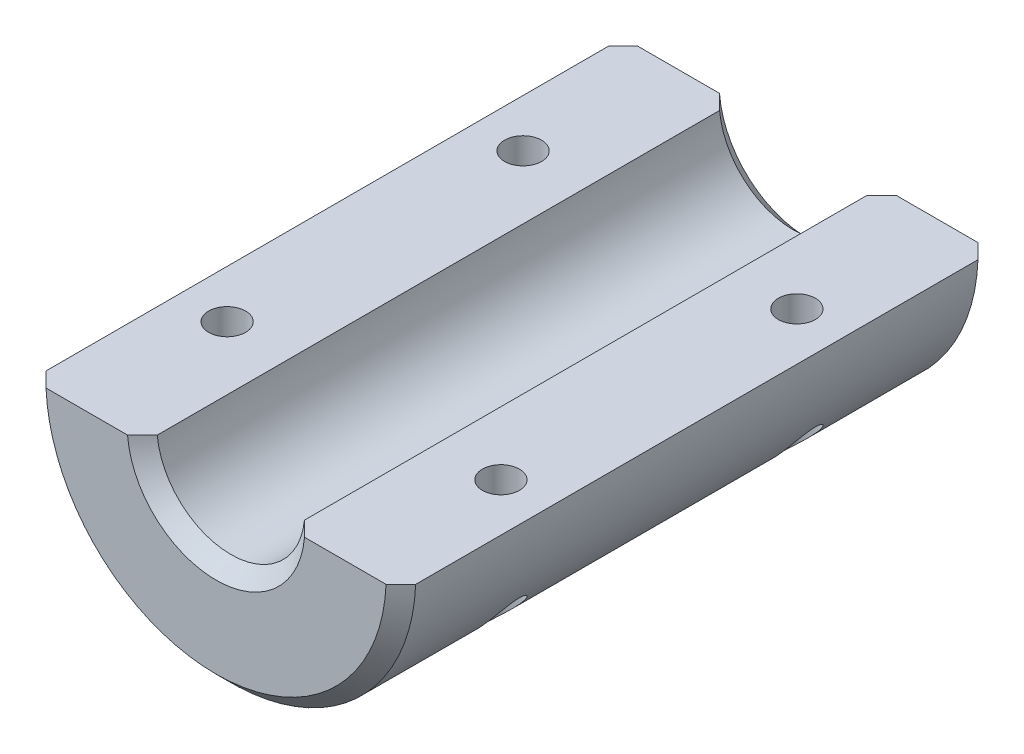
SolidWorks part; units mm, degrees
material "6061-T4 (SS)"
ref_plane "前视基准面" through (0, 0, 0) normal (0, 0, 1) x (1, 0, 0)
ref_plane "上视基准面" through (0, 0, 0) normal (0, 1, 0) x (1, 0, 0)
ref_plane "右视基准面" through (0, 0, 0) normal (1, 0, 0) x (0, 0, -1)
sketch "草图1" plane through (0, 0, 0) normal (0, 0, 1) x (1, 0, 0)
  line L0 (-24.98, -1) -> (-9.9499, -1)
  line L1 (9.9499, -1) -> (24.98, -1)
  arc A0 (-24.98, -1) -> (24.98, -1) centre (0, 0) ccw
  arc A1 (-9.9499, -1) -> (9.9499, -1) centre (0, 0) ccw
  dimension "D1" = 1
  dimension "D2" = 25
  dimension "D3" = 10
extrude "凸台-拉伸1" add sketch "草图1" along normal blind 80
hole_wizard "M6 螺纹孔1" positions "草图2" profile "草图3" tap size "M6" standard "GB" end condition through all
sketch "草图2" plane through (0, -1, 0) normal (0, 1, 0) x (1, 0, 0)
  line L1 (0, 0) -> (0, -67.6766) construction
  line L3 (-24.98, -40) -> (69.4253, -40) construction
  line L4 (-24.98, -80) -> (-24.98, 0) construction
  line L6 (-18.5, 0) -> (-18.5, -26.6939) construction
  line L9 (18.5, 0) -> (18.5, -26.6939) construction
  line L10 (18.5, -80) -> (18.5, -53.3061) construction
  line L11 (-18.5, -80) -> (-18.5, -53.3061) construction
  point P0 (-18.5, -20)
  point P24 (18.5, -20)
  point P29 (18.5, -60)
  point P30 (-18.5, -60)
  dimension "D1" = 40
  dimension "D2" = 37
sketch "草图3" plane through (-18.5, -1, 20) normal (1, 0, 0) x (0, 0, 1)
  line L0 (0, 0) -> (0, 24)
  line L1 (0, 24) -> (2.5, 24)
  line L2 (2.5, 24) -> (2.5, 0)
  line L5 (2.5, 0) -> (0, 0)
  line L11 (0, -6.35) -> (0, 107.95) construction
  dimension "通孔螺纹孔钻头直径" = 5
  dimension "通孔螺纹孔钻头深度" = 24
cosmetic thread "孔螺蚊线1" parameters "D2"=6
cosmetic thread "孔螺蚊线2" parameters "D2"=6
cosmetic thread "孔螺蚊线3" parameters "D2"=6
cosmetic thread "孔螺蚊线4" parameters "D2"=6
chamfer "倒角1" distance 2 angle 45 4 edges at (0, -25, 80) (0, -10, 80) (0, -25, 0) (0, -10, 0)
